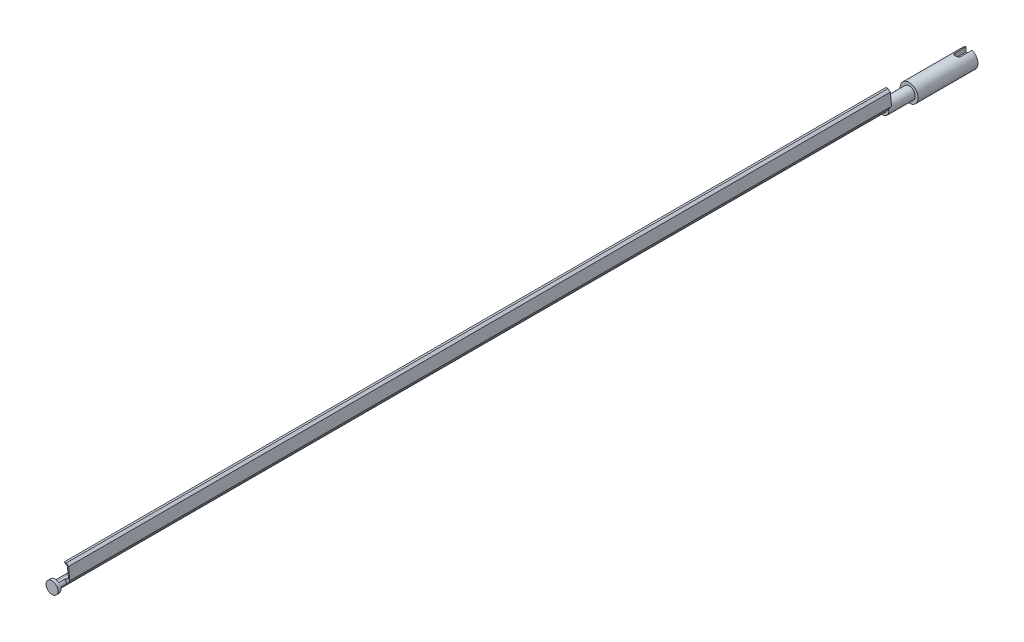
SolidWorks part; units mm, degrees
ref_plane "Front Plane" through (0, 0, 0) normal (0, 0, 1) x (1, 0, 0)
ref_plane "Top Plane" through (0, 0, 0) normal (0, 1, 0) x (1, 0, 0)
ref_plane "Right Plane" through (0, 0, 0) normal (1, 0, 0) x (0, 0, -1)
sketch "Sketch1" plane through (0, 0, 0) normal (0, 0, 1) x (1, 0, 0)
  circle A0 centre (0, 0) radius 100
  dimension "D1" = 200
extrude "Boss-Extrude1" add sketch "Sketch1" along normal blind 50
sketch "Sketch2" plane through (0, 0, 0) normal (0, 0, -1) x (-1, 0, 0)
  line L0 (-96.2334, 27.187) -> (-146.4287, 97.202)
  line L1 (-146.4287, 97.202) -> (-127.2387, 294.9434)
  line L2 (-127.2387, 294.9434) -> (-85.8554, 324.612)
  line L3 (-85.8554, 324.612) -> (-53.8157, 324.612)
  line L4 (-53.8157, 324.612) -> (-69.8355, 313.127)
  line L5 (-69.8355, 313.127) -> (-106.547, 286.8077)
  line L6 (-106.547, 286.8077) -> (-127.2387, 110.9598)
  line L7 (-127.2387, 110.9598) -> (-61.8256, 78.5977)
  line L8 (-61.8256, 78.5977) -> (0, 58.675)
  line L9 (-96.2334, 27.187) -> (-48.1874, -33.4774)
  circle A0 centre (0, 0) radius 100 construction
  arc A1 (-48.1874, -33.4774) -> (0, 58.675) centre (0, 0) ccw
extrude "Boss-Extrude2" add sketch "Sketch2" along normal blind 13824
sketch "Sketch3" plane through (0, 0, -13824) normal (0, 0, -1) x (-1, 0, 0)
  circle A0 centre (0, 0) radius 100
  dimension "D1" = 200
extrude "Boss-Extrude3" add sketch "Sketch3" along normal blind 440
sketch "Sketch4" plane through (0, 0, 0) normal (0, 0, 1) x (1, 0, 0)
  line L7 (96.2334, 27.187) -> (146.4287, 97.202)
  line L8 (146.4287, 97.202) -> (127.2387, 294.9434)
  line L9 (127.2387, 294.9434) -> (85.8554, 324.612)
  line L10 (85.8554, 324.612) -> (53.8157, 324.612)
  line L11 (53.8157, 324.612) -> (106.547, 286.8077)
  line L12 (106.547, 286.8077) -> (127.2387, 110.9598)
  line L13 (127.2387, 110.9598) -> (61.8256, 78.5977)
  line L14 (96.2334, 27.187) -> (146.4287, 97.202)
  line L15 (146.4287, 97.202) -> (127.2387, 294.9434)
  line L16 (127.2387, 294.9434) -> (85.8554, 324.612)
  line L17 (85.8554, 324.612) -> (53.8157, 324.612)
  line L18 (53.8157, 324.612) -> (106.547, 286.8077)
  line L19 (106.547, 286.8077) -> (127.2387, 110.9598)
  line L20 (127.2387, 110.9598) -> (61.8256, 78.5977)
  arc A1 (96.2334, 27.187) -> (61.8256, 78.5977) centre (0, 0) ccw
  arc A2 (96.2334, 27.187) -> (61.8256, 78.5977) centre (0, 0) ccw
  dimension "D1" = 0
extrude "Cut-Extrude1" cut sketch "Sketch4" against normal blind 100
sketch "Sketch6" plane through (0, 0, 50) normal (0, 0, 1) x (1, 0, 0)
  circle A0 centre (0, 0) radius 150
  dimension "D1" = 300
extrude "Boss-Extrude5" add sketch "Sketch6" along normal blind 2000
sketch "Sketch7" plane through (0, 0, 0) normal (0, 1, 0) x (1, 0, 0)
  line L0 (0, -1600) -> (0, -1900) construction
  line L1 (50, -1600) -> (50, -1900)
  line L2 (-50, -1600) -> (-50, -1900)
  line L3 (-150, -2050) -> (150, -2050) construction
  arc A0 (50, -1600) -> (-50, -1600) centre (0, -1600) ccw
  arc A1 (-50, -1900) -> (50, -1900) centre (0, -1900) ccw
  point P2 (0, -1750)
  dimension "D1" = 50
  dimension "D2" = 50
  dimension "D3" = 300
  dimension "D4" = 150
extrude "Cut-Extrude2" cut sketch "Sketch7" along normal blind 326
sketch "Sketch8" plane through (0, 0, 0) normal (0, 1, 0) x (1, 0, 0)
  line L2 (-50, -1600) -> (-50, -1900)
  line L3 (50, -1900) -> (50, -1600)
  line L4 (-50, -1600) -> (-50, -1900)
  line L5 (50, -1900) -> (50, -1600)
  arc A2 (50, -1600) -> (-50, -1600) centre (0, -1600) ccw
  arc A3 (-50, -1900) -> (50, -1900) centre (0, -1900) ccw
  arc A4 (50, -1600) -> (-50, -1600) centre (0, -1600) ccw
  arc A5 (-50, -1900) -> (50, -1900) centre (0, -1900) ccw
  dimension "D1" = 0
extrude "Boss-Extrude6" add sketch "Sketch8" along normal blind 75
sketch "Sketch9" plane through (0, 0, -14264) normal (0, 0, -1) x (-1, 0, 0)
  circle A0 centre (0, 0) radius 150
  dimension "D1" = 300
extrude "Boss-Extrude7" add sketch "Sketch9" along normal blind 1000
sketch "Sketch10" plane through (0, 0, 0) normal (0, 1, 0) x (1, 0, 0)
  line L0 (0, 15384) -> (0, 15084) construction
  line L1 (50, 15384) -> (50, 15084)
  line L2 (-50, 15384) -> (-50, 15084)
  line L3 (150, 15264) -> (-150, 15264) construction
  arc A0 (50, 15384) -> (-50, 15384) centre (0, 15384) ccw
  arc A1 (-50, 15084) -> (50, 15084) centre (0, 15084) ccw
  point P2 (0, 15234)
  dimension "D1" = 120
  dimension "D2" = 300
  dimension "D3" = 100
extrude "Cut-Extrude3" cut sketch "Sketch10" along normal blind 300 from offset 65
sketch "Sketch11" plane through (0, 0, 0) normal (0, 1, 0) x (1, 0, 0)
  line L1 (150, -50) -> (-150, -50)
  line L2 (150, -50) -> (150, -2050)
  line L3 (150, -2050) -> (-150, -2050)
  line L4 (-150, -50) -> (-150, -2050)
extrude "Cut-Extrude4" cut sketch "Sketch11" against normal mid plane 500
